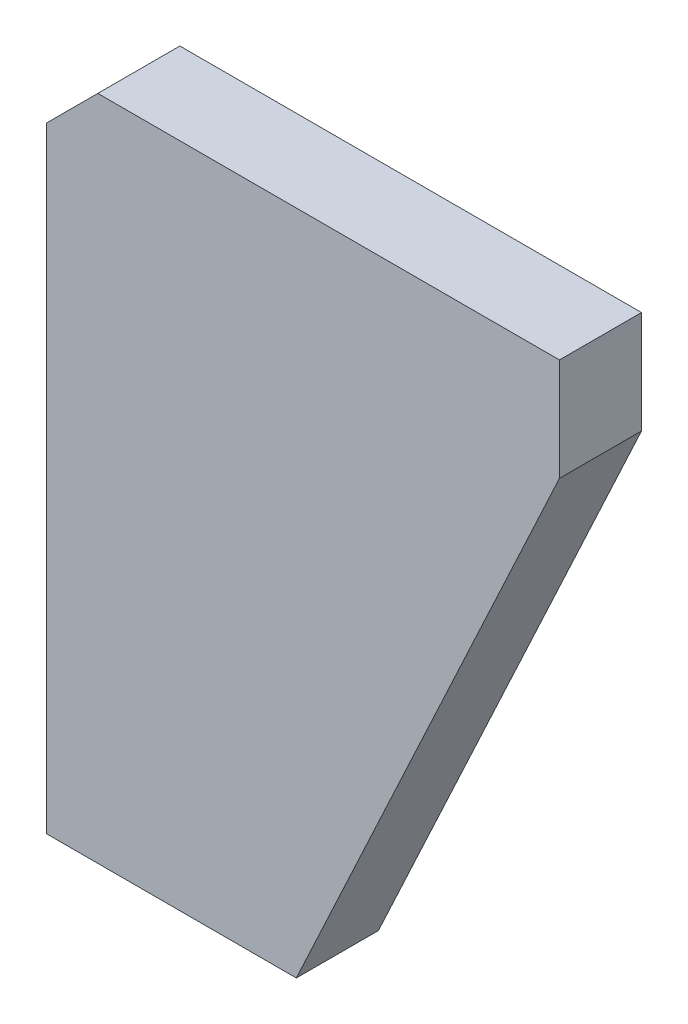
SolidWorks part; units mm, degrees
material "普通碳钢"
ref_plane "Front Plane" through (0, 0, 0) normal (0, 0, 1) x (1, 0, 0)
ref_plane "Top Plane" through (0, 0, 0) normal (0, 1, 0) x (1, 0, 0)
ref_plane "Right Plane" through (0, 0, 0) normal (1, 0, 0) x (0, 0, -1)
sketch "Sketch1" plane through (0, 0, 0) normal (0, 0, 1) x (1, 0, 0)
  line L4 (50, 65) -> (0, 65)
  line L6 (0, 65) -> (0, 0)
  line L7 (50, 55) -> (24.3531, 0)
  line L8 (50, 65) -> (50, 55)
  line L9 (0, 0) -> (24.3531, 0)
  dimension "D1" = 65
  dimension "D2" = 10
  dimension "D3" = 50
  dimension "D4" = 65
extrude "Boss-Extrude1" add sketch "Sketch1" along normal blind 8
chamfer "Chamfer1" distance 5 angle 45 1 edges at (0, 65, 4)
